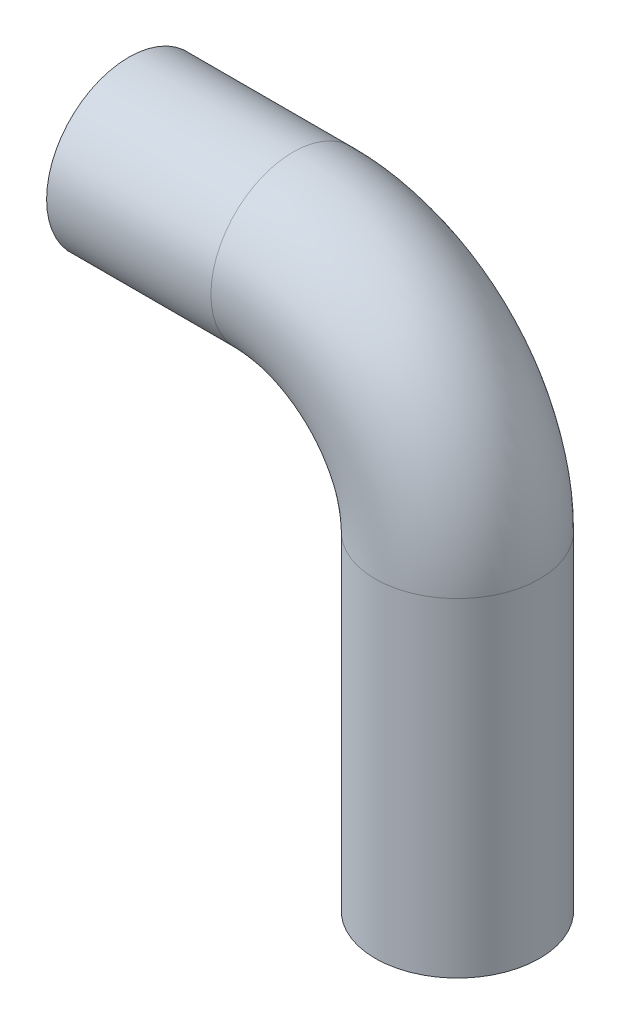
from build123d import *

# Parameters (mm, degrees)
SKETCH2_R   = 5
SKETCH2_R_2 = 4


with BuildPart() as part:
    # Sweep1: sweep along a path in Sketch1
    with BuildLine(Plane.XY) as sweep1_path:
        Line((0, 0), (10, 0))
        ThreePointArc((10, 0), (17.071067812, -2.928932188), (20, -10))
        Line((20, -10), (20, -30))
    # Sketch2 → Sweep1 (sweep)
    with BuildSketch(Plane(origin=(0, 0, 0), x_dir=(0, 0, -1), z_dir=(1, 0, 0))):
        Circle(SKETCH2_R)
        Circle(SKETCH2_R_2, mode=Mode.SUBTRACT)
    sweep(path=sweep1_path.line)


solid = part.part
